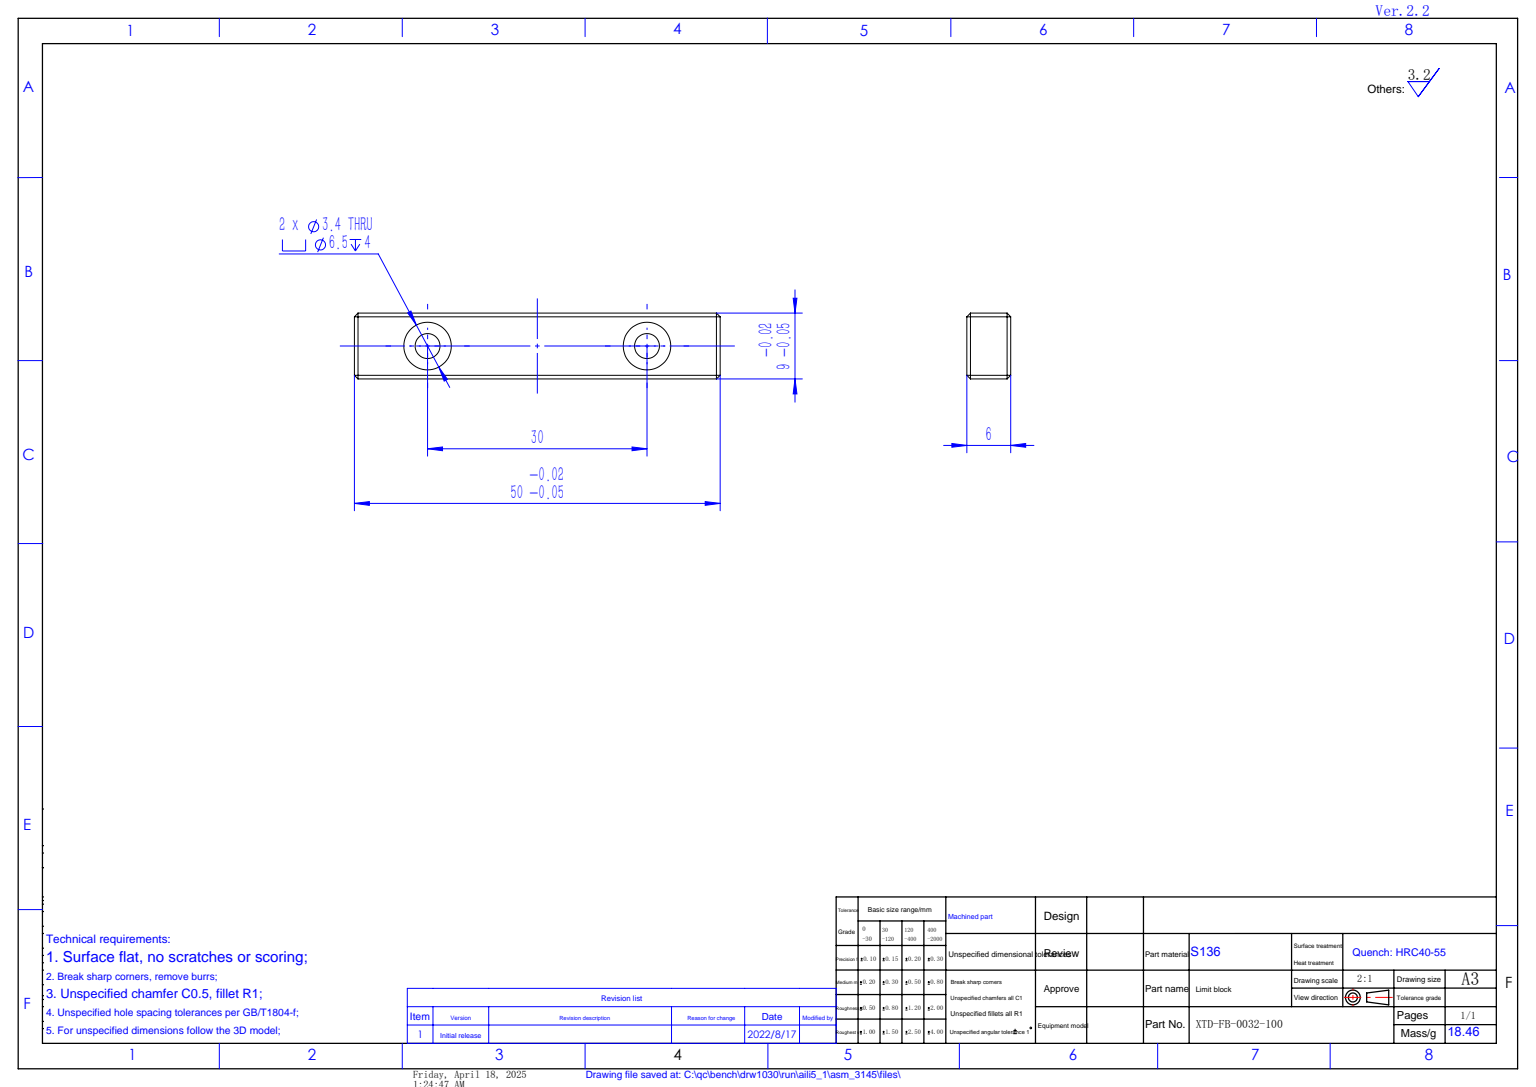
SolidWorks part; units mm, degrees
material "S136"
ref_plane "前视基准面" through (0, 0, 0) normal (0, 0, 1) x (1, 0, 0)
ref_plane "上视基准面" through (0, 0, 0) normal (0, 1, 0) x (1, 0, 0)
ref_plane "右视基准面" through (0, 0, 0) normal (1, 0, 0) x (0, 0, -1)
sketch "草图1" plane through (0, 0, 0) normal (0, 1, 0) x (1, 0, 0)
  line L1 (25, -4.5) -> (-25, -4.5)
  line L2 (25, -4.5) -> (25, 4.5)
  line L3 (25, 4.5) -> (-25, 4.5)
  line L4 (-25, -4.5) -> (-25, 4.5)
  line L5 (25, -4.5) -> (-25, 4.5) construction
  line L6 (25, 4.5) -> (-25, -4.5) construction
  point P0 (0, 0)
  dimension "D1" = 50
  dimension "D2" = 9
extrude "凸台-拉伸1" add sketch "草图1" along normal blind 6
chamfer "倒角1" distance 0.5 angle 45 12 edges at (25, 3, 4.5) (25, 3, -4.5) (-25, 3, -4.5) (0, 0, 4.5) (25, 0, 0) (0, 0, -4.5) (-25, 0, 0) (-25, 3, 4.5) (0, 6, -4.5) (25, 6, 0) (0, 6, 4.5) (-25, 6, 0)
hole_wizard "M3 六角凹头螺钉的柱形沉头孔1" positions "草图2" profile "草图3" counterbore size "M3" standard "ISO" end condition through all
sketch "草图2" plane through (0, 6, 0) normal (0, 1, 0) x (1, 0, 0)
  line L0 (-15, 0) -> (15, 0) construction
  line L1 (0, 0) -> (0, -4.5) construction
  line L2 (24.5, -4.5) -> (-24.5, -4.5) construction
  line L4 (15, 0) -> (25, 0) construction
  line L5 (25, 4) -> (25, -4) construction
  point P0 (-15, 0)
  point P2 (15, 0)
  dimension "D1" = 30
sketch "草图3" plane through (-15, 6, 0) normal (1, 0, 0) x (0, 0, 1)
  line L0 (0, 0) -> (0, 6)
  line L1 (0, 6) -> (1.7, 6)
  line L3 (1.7, 6) -> (1.7, 4)
  line L4 (1.7, 4) -> (3.25, 4)
  line L5 (3.25, 4) -> (3.25, 0)
  line L7 (3.25, 0) -> (0, 0)
  line L11 (0, -6.35) -> (0, 107.95) construction
  dimension "通孔孔直径" = 3.4
  dimension "通孔孔深度" = 6
  dimension "柱形沉头孔直径" = 6.5
  dimension "柱形沉头孔深度" = 4
